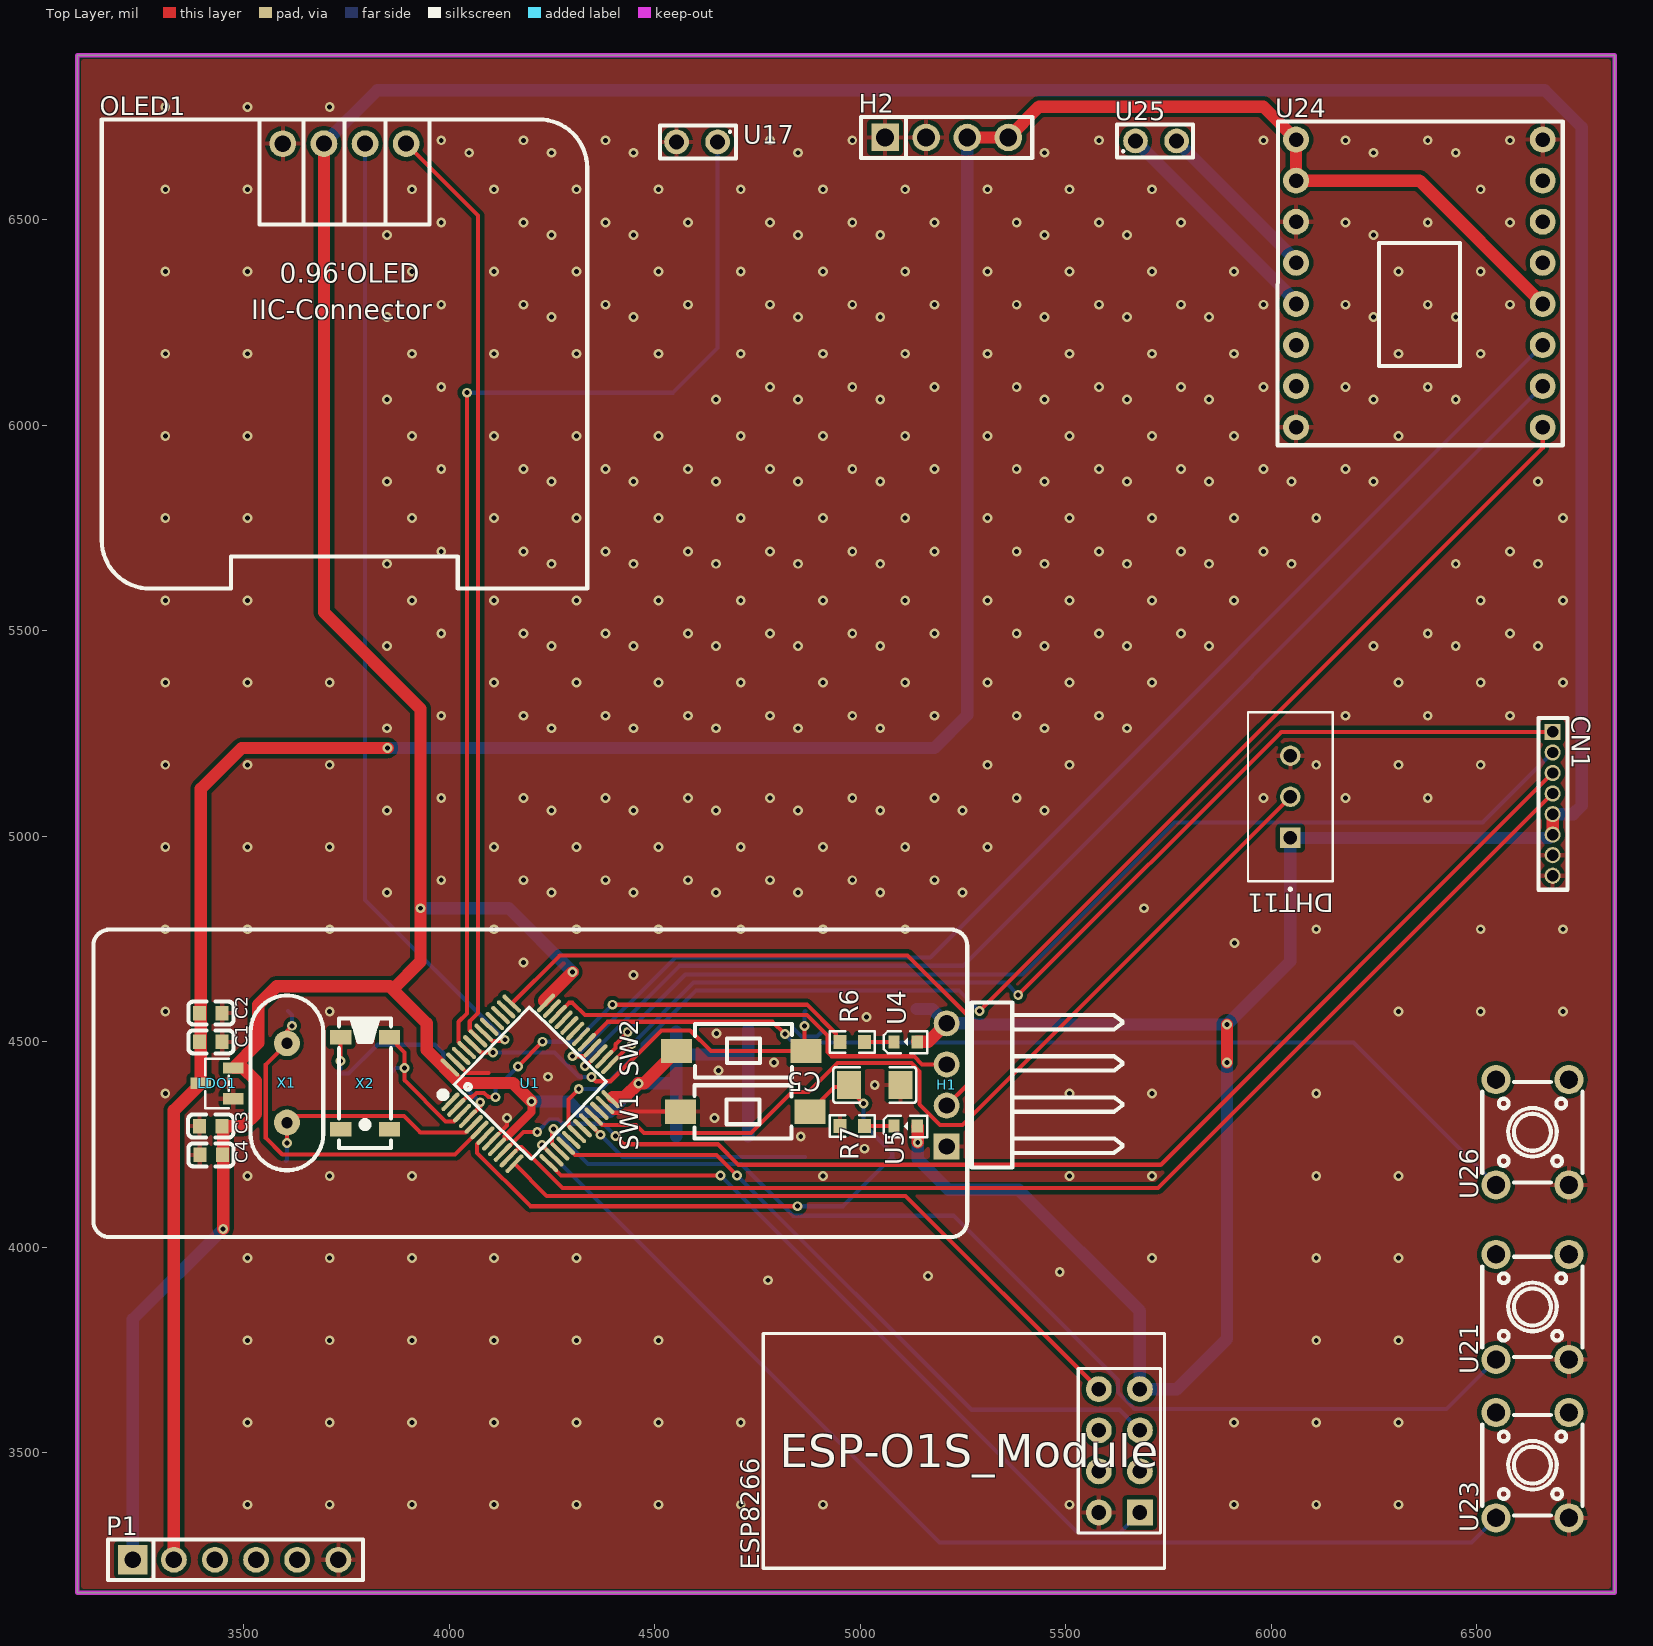
[diagram p0: Top Layer view]
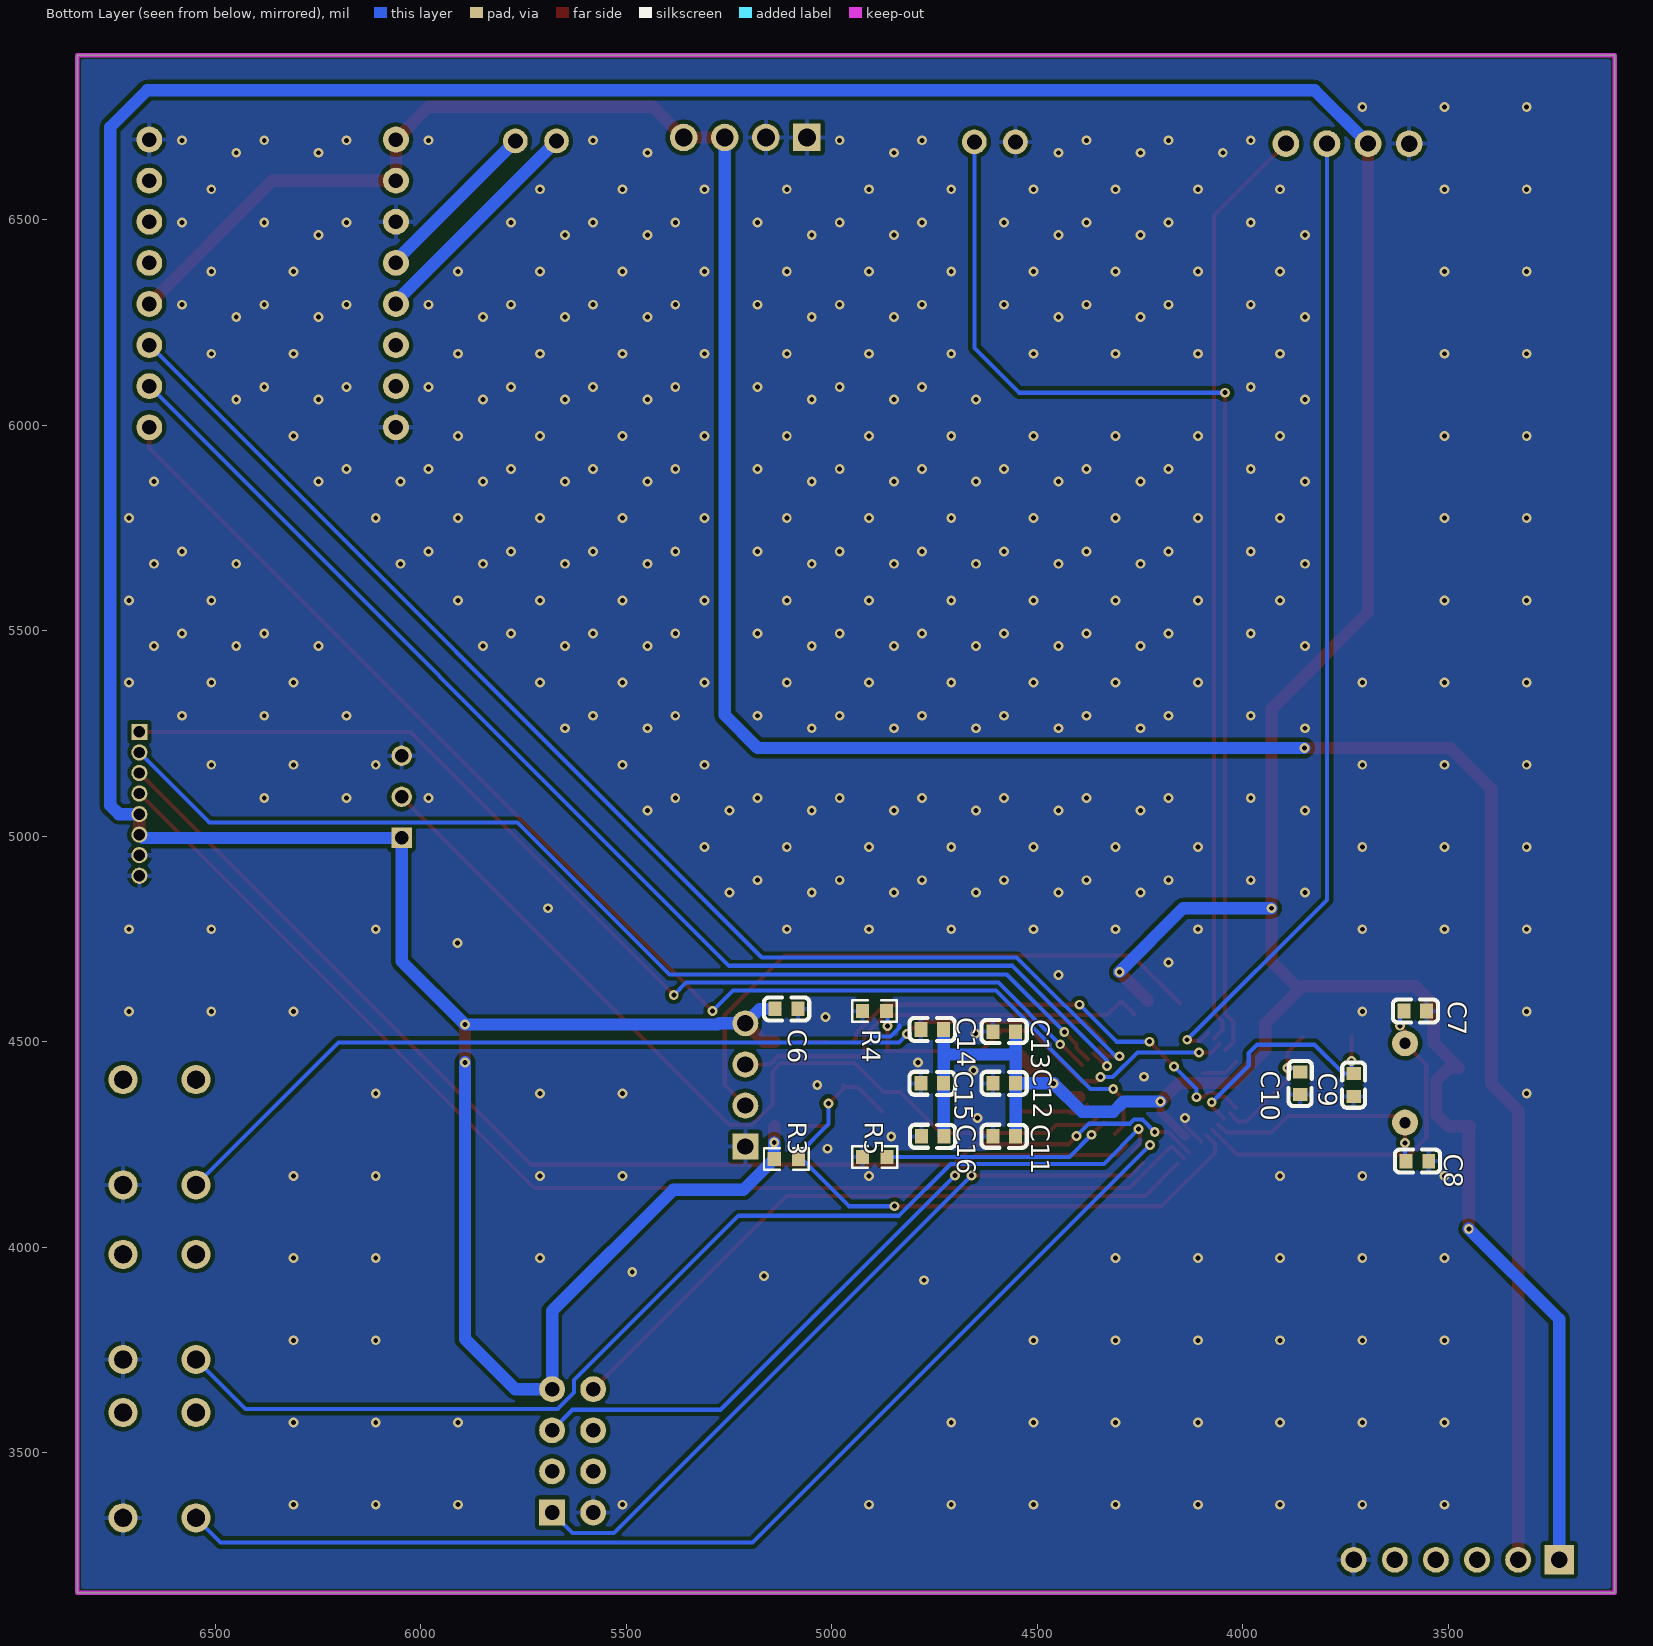
[diagram p1: Bottom Layer view, seen from below]
# Altium PCB MISC89131.pcbdoc
Units mil, origin at the board's own origin, x right, y up, seen from the top; angles counter-clockwise.
Board outline 3740.16 x 3740.16 mil, 2 copper layers (Top Layer, Bottom Layer), stack 62.206 mil thick; 42 components, 47 nets, 176 pads, 453 vias.

## Layer stack, top to bottom
Top Solder Mask Layer: solder mask 0.394, Dk 3.3
Top Layer: signal copper 1.379
Dielectric1: surface 59.449, FR4, Dk 4.5
Bottom Layer: signal copper 1.378
Bottom Solder Mask Layer: solder mask 0.394, Dk 3.3

## Board outline
3095,6900 3095,3159.84 6835.16,3159.84 6835.16,6900

## Design rules (kind name [scope] priority, off if disabled: settings)
BoardOutlineClearance copperThickness2oz_1 [All] p2: genericclearance=7.99 ignorepadtopadclearanceinfootprint=FALSE except(0: Arc-SplitContinuation Track-SplitContinuation SMDPad-SplitContinuation THPad-SplitContinuation Via-SplitContinuation Fill-SplitContinuation Region-SplitContinuation Poly-SplitContinuation Text-SplitContinuation Hole-SplitContinuation; 5.98: Arc-CutoutEdge Track-CutoutEdge SMDPad-CutoutEdge THPad-CutoutEdge Via-CutoutEdge Text-CutoutEdge; 6.89: Hole-OutlineEdge Hole-CutoutEdge; 10: Poly-OutlineEdge Poly-CutoutEdge; 11.81: Arc-OutlineEdge Track-OutlineEdge SMDPad-OutlineEdge THPad-OutlineEdge Via-OutlineEdge Fill-OutlineEdge Region-OutlineEdge Text-OutlineEdge Fill-CutoutEdge Region-CutoutEdge)
BoardOutlineClearance Plane_innerPlane_1 [All] p4 off: genericclearance=4.02 ignorepadtopadclearanceinfootprint=FALSE except(0: Arc-SplitContinuation Track-SplitContinuation SMDPad-SplitContinuation THPad-SplitContinuation Via-SplitContinuation Fill-SplitContinuation Region-SplitContinuation Poly-SplitContinuation Text-SplitContinuation Hole-SplitContinuation; 5.98: Arc-CutoutEdge Track-CutoutEdge SMDPad-CutoutEdge THPad-CutoutEdge Via-CutoutEdge Text-CutoutEdge; 6.89: Hole-OutlineEdge Hole-CutoutEdge; 10: Poly-OutlineEdge Poly-CutoutEdge; 11.81: Arc-OutlineEdge Track-OutlineEdge SMDPad-OutlineEdge THPad-OutlineEdge Via-OutlineEdge Fill-OutlineEdge Region-OutlineEdge Text-OutlineEdge Fill-CutoutEdge Region-CutoutEdge)
BoardOutlineClearance Copper_copperRegion_1 [All] p6 off: genericclearance=4.02 ignorepadtopadclearanceinfootprint=FALSE except(0: Arc-SplitContinuation Track-SplitContinuation SMDPad-SplitContinuation THPad-SplitContinuation Via-SplitContinuation Fill-SplitContinuation Region-SplitContinuation Poly-SplitContinuation Text-SplitContinuation Hole-SplitContinuation; 5.98: Arc-CutoutEdge Track-CutoutEdge SMDPad-CutoutEdge THPad-CutoutEdge Via-CutoutEdge Text-CutoutEdge; 6.89: Hole-OutlineEdge Hole-CutoutEdge; 10: Poly-OutlineEdge Poly-CutoutEdge; 11.81: Arc-OutlineEdge Track-OutlineEdge SMDPad-OutlineEdge THPad-OutlineEdge Via-OutlineEdge Fill-OutlineEdge Region-OutlineEdge Text-OutlineEdge Fill-CutoutEdge Region-CutoutEdge)
BoardOutlineClearance copperThickness1oz_1 [All] p8: genericclearance=4.02 ignorepadtopadclearanceinfootprint=FALSE except(0: Arc-SplitContinuation Track-SplitContinuation SMDPad-SplitContinuation THPad-SplitContinuation Via-SplitContinuation Fill-SplitContinuation Region-SplitContinuation Poly-SplitContinuation Text-SplitContinuation Hole-SplitContinuation; 5.98: Arc-CutoutEdge Track-CutoutEdge SMDPad-CutoutEdge THPad-CutoutEdge Via-CutoutEdge Text-CutoutEdge; 6.89: Hole-OutlineEdge Hole-CutoutEdge; 10: Poly-OutlineEdge Poly-CutoutEdge; 11.81: Arc-OutlineEdge Track-OutlineEdge SMDPad-OutlineEdge THPad-OutlineEdge Via-OutlineEdge Fill-OutlineEdge Region-OutlineEdge Text-OutlineEdge Fill-CutoutEdge Region-CutoutEdge)
Clearance copperThickness2oz [(InNet('+5V'))] p1: gap=7.99 ignorepadtopadclearanceinfootprint=FALSE except(5.98: SMDPad-Track SMDPad-SMDPad THPad-Track SMDPad-THPad THPad-THPad Track-Via SMDPad-Via THPad-Via Via-Via Fill-SMDPad Region-SMDPad Fill-THPad Region-THPad Fill-Via Region-Via Fill-Fill Fill-Region Region-Region Arc-Track Arc-SMDPad Arc-THPad Arc-Via Fill-Arc Region-Arc Arc-Arc Text-Track SMDPad-Text Text-THPad Text-Via Fill-Text Region-Text Arc-Text Text-Text; 6.89: Hole-Track Hole-SMDPad Hole-THPad Hole-Via Fill-Hole Region-Hole Hole-Arc Hole-Text; 10: Poly-Track Poly-SMDPad Poly-THPad Poly-Via Poly-Fill Poly-Region Poly-Poly Poly-Arc Poly-Text Poly-Hole; 11.81: Fill-Track Region-Track)
Clearance Plane_innerPlane [All] p3 off: gap=4.02 ignorepadtopadclearanceinfootprint=FALSE except(5.98: SMDPad-Track SMDPad-SMDPad THPad-Track SMDPad-THPad THPad-THPad Track-Via SMDPad-Via THPad-Via Via-Via Fill-SMDPad Region-SMDPad Fill-THPad Region-THPad Fill-Via Region-Via Fill-Fill Fill-Region Region-Region Arc-Track Arc-SMDPad Arc-THPad Arc-Via Fill-Arc Region-Arc Arc-Arc Text-Track SMDPad-Text Text-THPad Text-Via Fill-Text Region-Text Arc-Text Text-Text; 6.89: Hole-Track Hole-SMDPad Hole-THPad Hole-Via Fill-Hole Region-Hole Hole-Arc Hole-Text; 10: Poly-Track Poly-SMDPad Poly-THPad Poly-Via Poly-Fill Poly-Region Poly-Poly Poly-Arc Poly-Text Poly-Hole; 11.81: Fill-Track Region-Track)
Clearance Copper_copperRegion [All] p5 off: gap=4.02 ignorepadtopadclearanceinfootprint=FALSE except(5.98: SMDPad-Track SMDPad-SMDPad THPad-Track SMDPad-THPad THPad-THPad Track-Via SMDPad-Via THPad-Via Via-Via Fill-SMDPad Region-SMDPad Fill-THPad Region-THPad Fill-Via Region-Via Fill-Fill Fill-Region Region-Region Arc-Track Arc-SMDPad Arc-THPad Arc-Via Fill-Arc Region-Arc Arc-Arc Text-Track SMDPad-Text Text-THPad Text-Via Fill-Text Region-Text Arc-Text Text-Text; 6.89: Hole-Track Hole-SMDPad Hole-THPad Hole-Via Fill-Hole Region-Hole Hole-Arc Hole-Text; 10: Poly-Track Poly-SMDPad Poly-THPad Poly-Via Poly-Fill Poly-Region Poly-Poly Poly-Arc Poly-Text Poly-Hole; 11.81: Fill-Track Region-Track)
Clearance copperThickness1oz [All] p7: gap=4.02 ignorepadtopadclearanceinfootprint=FALSE except(5.98: SMDPad-Track SMDPad-SMDPad THPad-Track SMDPad-THPad THPad-THPad Track-Via SMDPad-Via THPad-Via Via-Via Fill-SMDPad Region-SMDPad Fill-THPad Region-THPad Fill-Via Region-Via Fill-Fill Fill-Region Region-Region Arc-Track Arc-SMDPad Arc-THPad Arc-Via Fill-Arc Region-Arc Arc-Arc Text-Track SMDPad-Text Text-THPad Text-Via Fill-Text Region-Text Arc-Text Text-Text; 6.89: Hole-Track Hole-SMDPad Hole-THPad Hole-Via Fill-Hole Region-Hole Hole-Arc Hole-Text; 10: Poly-Track Poly-SMDPad Poly-THPad Poly-Via Poly-Fill Poly-Region Poly-Poly Poly-Arc Poly-Text Poly-Hole; 11.81: Fill-Track Region-Track)
DiffPairsRouting differentialPair [All] p1: maxlimit=6 minlimit=6 mostfreqgap=6 toplayer_minwidth=5 toplayer_prefwidth=10 toplayer_maxwidth=100 toplayer_mingap=6 toplayer_prefgap=6 toplayer_maxgap=6 bottomlayer_minwidth=5 bottomlayer_prefwidth=10 bottomlayer_maxwidth=100 bottomlayer_mingap=6 bottomlayer_prefgap=6 bottomlayer_maxgap=6 maxuncoupledlength=10
HoleToHoleClearance otherClearance [All] p1: gap=11.81 allowstackedmicrovias=TRUE
Length netLength [All] p1: minlimit=0 maxlimit=0
PasteMaskExpansion pasteMaskExpansion [All] p1: expansion=0
PlaneConnect innerPlane [All] p1: planeconnectstyle=Relief reliefexpansion=20 reliefentries=4 reliefconductorwidth=10 reliefairgap=10
PolygonConnect copperRegion [All] p1: connectstyle=Relief reliefconductorwidth=10 reliefentries=4 polygonreliefangle="90 Angle" airgapwidth=10 via.connectstyle=Relief via.reliefconductorwidth=10 via.reliefentries=4 via.polygonreliefangle="90 Angle" via.airgapwidth=10
RoutingVias viaSize [All] p1: holewidth=12.01 width=24.02 viastyle="Through Hole" minholewidth=11.81 minwidth=19.68 maxholewidth=248.03 maxwidth=393.7
SolderMaskExpansion solderMaskExpansion [IsVia] p1: expansion=-1000 istentingtop=TRUE
SolderMaskExpansion solderMaskExpansion [All] p2: expansion=2.01 istentingtop=FALSE
Width copperThickness2oz_2 [(InNet('+5V'))] p1: maxlimit=100 minlimit=15 preferedwidth=15
Width copperThickness1oz_2 [All] p2: maxlimit=100 minlimit=5 preferedwidth=10

## Components (designator, comment, footprint, x,y, rotation, side; value= is the part's Value field where it differs from the comment)
C1 "10uF" C0603 3420,4500 r180 top
C2 "100nF" C0603 3420,4570 r180 top
C3 "100nF" C0603 3420,4295 r0 top
C4 "10uF" C0603 3420.61,4224.79 r0 top
C5 "100uF" C1206 5035,4395 r180 top
C6 "100nF" C0603 5109.76,4580 r0 bottom
C7 "20pF" C0603 3580,4575 r0 bottom
C8 "20pF" C0603 3575,4210 r0 bottom
C9 "20pF" C0603 3730,4395 r90 bottom
C10 "20pF" C0603 3860,4399.02 r90 bottom
C11 "100nF" C0603 4580,4270 r180 bottom
C12 "100nF" C0603 4580,4399.02 r180 bottom
C13 "100nF" C0603 4580,4525 r180 bottom
C14 "100nF" C0603 4755,4530 r180 bottom
C15 "100nF" C0603 4755,4399.02 r180 bottom
C16 "4.7nF" C0603 4754.05,4270 r180 bottom
CN1 "2.0mm*8P female header" HDR-TH_8P-P1.27_2.0MM-8P 6684.01,5079.02 r270 top
DHT11 "" PIN3直插DHT11 6135,5085 r180 top
ESP8266 "" ESP8266-01S_Module 5630,3505 r90 top
H1 "A254AD-WD04P" HDR-TH_4P-P2.54-H-M-W10.2 5210,4395 r90 top
H2 "4P" HDR-TH_4P-P2.54-V-M-3 5210,6700 r0 top
LDO1 "SC662K-3.3V" SOT-23-3_L2.9-W1.3-P1.90-LS2.4-BR 3435,4399.02 r0 top
OLED1 "" 0.96OLED_4P 3745,6685 r0 top
P1 "MINI USB power input module" HDR-TH_6P-P2.54-V-F 3480,3240 r0 top
R3 "1kΩ" R0603 5110,4215 r0 bottom
R4 "10kΩ" R0603 4895.68,4575 r180 bottom
R5 "10kΩ" R0603 4895,4220 r180 bottom
R6 "510Ω" R0603 4980,4500 r180 top
R7 "510Ω" R0603 4980,4295 r180 top
SW1 "TS-1101-C-W" SW-SMD_L6.0-W3.3-LS8.0 4720,4330.12 r0 top
SW2 "TS-1101-C-W" SW-SMD_L6.0-W3.3-LS8.0 4710,4477.76 r180 top
U1 "STM32F103C8T6" LQFP-48_L7.0-W7.0-P0.50-LS9.0-BL 4197.01,4399.02 r316 top
U4 "42-51/GHC-YW2X2K/3T" LED-SMD_L1.6-W0.8-FD_GREEN-1 5110,4500 r180 top
U5 "42-51/GHC-YW2X2K/3T" LED-SMD_L1.6-W0.8-FD_GREEN-1 5110,4295 r180 top
U17 "" 2p排针 4652.81,6689.16 r180 top
U21 "UP" KEY-TH_4P复位按键 6635,3855 r90 top
U23 "DOWN" KEY-TH_4P复位按键 6635,3470 r90 top
U24 "" TB6612电机驱动 6360,6345 r0 top
U25 "" 2p排针 5669.39,6691.55 r0 top
U26 "UP" KEY-TH_4P复位按键 6635,4280 r90 top
X1 "8MHz" OSC-TH_L10.0-W4.5-P5.00 3605,4400 r180 top
X2 "32.768kHz" MC-306_4P-L8.0-W3.2-P5.5-BL 3795,4399.02 r270 top

## Footprints (in the part's own frame and the unit in brackets; to place one, negate y for a bottom-side part, rotate by r counter-clockwise, add the part's x,y. Pads: shape width x height; smd on the part's side, far side on the other; paste and mask are expansions set on the pad)
0.96OLED_4P [mm]
  round 1.65 hole 1 copper offset 0,0: 1(-3.81,-0.001) 2(-1.27,0.002) 3(1.27,0.002) 4(3.81,0.002)
  silkscreen extent -15,-27.5 15,1.5
2p排针 [mil]
  round 60 hole 36: 1(0,0) 2(100,0)
  silkscreen extent -45,-40 140,40
C0603 [mm]
  rect 0.8x0.9 smd: 1(-0.7,0) 2(0.7,0)
  silkscreen extent -1.41,-0.71 1.39,0.72
C1206 [mm]
  rect 1.485x1.728 smd paste-100 mask+0.051: 1(-1.593,0) 2(1.593,0)
  silkscreen extent -2.56,-1.09 2.56,1.09
ESP8266-01S_Module [mm]
  rect 1.6x1.6 hole 0.9: 1(-3.81,-1.27)
  round 1.6 hole 0.9: 2(-3.81,1.27) 3(-1.27,-1.27) 4(-1.27,1.27) 5(1.27,-1.27) 6(1.27,1.27) 7(3.81,-1.27) 8(3.81,1.27)
  silkscreen extent -7.25,-2.79 7.25,22.01
HDR-TH_4P-P2.54-H-M-W10.2 [mm]
  rect 1.6x1.6 hole 1: 1(-3.81,0)
  round 1.6 hole 1: 2(-1.27,0) 3(1.27,0) 4(3.81,0)
  silkscreen extent -5.1,-10.85 5.1,-1.55
HDR-TH_4P-P2.54-V-M-3 [mil]
  rect 66.9x66.9 hole 43.3 paste+0 mask+2: 1(-150,0)
  round 66.9 hole 43.3 paste+0 mask+2: 2(-50,0) 3(50,0) 4(150,0)
  silkscreen extent -208,-50 208,50
HDR-TH_6P-P2.54-V-F [mm]
  rect 1.8x1.8 hole 1.02: 1(-6.35,0)
  round 1.6 hole 1.02: 2(-3.81,0) 3(-1.27,0) 4(1.27,0) 5(3.81,0) 6(6.35,0)
  silkscreen extent -7.87,-1.25 7.87,1.25
HDR-TH_8P-P1.27_2.0MM-8P [mm]
  rect 1x1 hole 0.7: 1(-4.445,0)
  round 1 hole 0.7: 2(-3.175,0) 3(-1.905,0) 4(-0.635,0) 5(0.635,0) 6(1.905,0) 7(3.175,0) 8(4.445,0)
  silkscreen extent -5.31,-0.87 5.31,0.92
KEY-TH_4P复位按键 [mm]
  round 1.8 hole 1.1 slot 1.105 at 0 deg: 1(-3.251,2.25) 2(3.251,2.25) 3(-3.251,-2.25) 4(3.251,-2.25)
  silkscreen extent -3.1,-3.1 3.1,3.1
LED-SMD_L1.6-W0.8-FD_GREEN-1 [mm]
  rect 0.7x0.8 smd: 1(-0.715,0) 2(0.715,0)
  silkscreen extent -1.35,-0.65 1.35,0.7
LQFP-48_L7.0-W7.0-P0.50-LS9.0-BL [mm]
  oval 0.27x1.5 smd rot 179.96 paste+0 mask+0.05: 1(-2.753,-4.248) 2(-2.253,-4.248) 3(-1.753,-4.249) 4(-1.253,-4.249) 5(-0.753,-4.249) 6(-0.253,-4.25) 7(0.247,-4.25) 8(0.747,-4.25) 9(1.247,-4.251) 10(1.747,-4.251) 11(2.247,-4.251) 12(2.747,-4.252) 25(2.753,4.248) 26(2.253,4.248) 27(1.753,4.249) 28(1.253,4.249) 29(0.753,4.249) 30(0.253,4.25) 31(-0.247,4.25) 32(-0.747,4.25) 33(-1.247,4.251) 34(-1.747,4.251) 35(-2.247,4.251) 36(-2.747,4.252)
  oval 1.5x0.27 smd rot 179.96 paste+0 mask+0.05: 13(4.248,-2.753) 14(4.248,-2.253) 15(4.249,-1.753) 16(4.249,-1.253) 17(4.249,-0.753) 18(4.25,-0.253) 19(4.25,0.247) 20(4.25,0.747) 21(4.251,1.247) 22(4.251,1.747) 23(4.251,2.247) 24(4.252,2.747) 37(-4.248,2.753) 38(-4.248,2.253) 39(-4.249,1.753) 40(-4.249,1.253) 41(-4.249,0.753) 42(-4.25,0.253) 43(-4.25,-0.247) 44(-4.25,-0.747) 45(-4.251,-1.247) 46(-4.251,-1.747) 47(-4.251,-2.247) 48(-4.252,-2.747)
  silkscreen extent -3.59,-4.46 3.3,3.34
MC-306_4P-L8.0-W3.2-P5.5-BL [mm]
  rect 0.9x1.3 smd: 1(-2.85,-1.5) 2(2.85,-1.5) 3(2.85,1.5) 4(-2.85,1.5)
  silkscreen extent -4,-1.6 4,1.6
OSC-TH_L10.0-W4.5-P5.00 [mm]
  round 1.6 hole 0.7: 1(0,2.45) 2(0,-2.45)
  silkscreen extent -2.25,-5.39 2.25,5.39
PIN3直插DHT11 [mm]
  rect 1.26x1.26 hole 0.84: 1(2.26,2.26)
  round 1.26 hole 0.84: 2(2.26,-0.28) 3(2.26,-2.82)
  silkscreen extent -0.36,-5.51 4.88,5.51
R0603 [mil]
  rect 31.75x34.02 smd paste-3937.01 mask+2: 1(-29.66,0) 2(29.66,0)
  silkscreen extent -55,-26 55,26
SOT-23-3_L2.9-W1.3-P1.90-LS2.4-BR [mm]
  rect 1.25x0.7 smd: 1(1,-0.95) 2(1,0.95) 3(-1,0)
  silkscreen extent -0.73,-1.53 0.73,1.53
SW-SMD_L6.0-W3.3-LS8.0 [mm]
  rect 1.9x1.5 smd: 1(-4,0) 2(4,0)
  silkscreen extent -3.14,-1.67 2.86,1.63
TB6612电机驱动 [mm]
  round 1.6 hole 0.9 paste+0 mask+0.051: 1(-7.62,8.89) 2(-7.62,6.35) 3(-7.62,3.81) 4(-7.62,1.27) 5(-7.62,-1.27) 6(-7.62,-3.81) 7(-7.62,-6.35) 8(-7.62,-8.89) 9(7.62,8.89) 10(7.62,6.35) 11(7.62,3.81) 12(7.62,1.27) 13(7.62,-1.27) 14(7.62,-3.81) 15(7.62,-6.35) 16(7.62,-8.89)
  silkscreen extent -8.77,-10 8.86,10

## Via types
v1: diameter 24.02, hole 12, Top Layer to Bottom Layer, 453 vias

## Nets (pads, with @x,y where several pads share a name; then routed paths per layer and width w, separated by ;. In a path a pad name is that pad's centre, name@x,y a point inside that pad or via, vN(x,y) a via of type N, cw(c..) or ccw(c..) an arc to the next point about the centre after c; other vN are vias at no path point)
3V3: C3.2 C4.2 C6.2 C11.2 C12.2 C13.2 C14.2 C15.2 C16.2 CN1.5 CN1.6 DHT11.1 ESP8266.7 H1.4 LDO1.2 OLED1.2 P1.1 R3.2 SW2.2 U1.9 U1.24 U1.36 U1.48 U4.1 U5.1 | length 15462.2
  Top Layer w20: 4139.99,4269.54 4200,4329.55 v1(4200,4355)
  Top Layer w30: v1(3450,4045) 3450,4292.56 C3.2 3500,4295 3529.6,4324.6 3529.6,4405.4 3498.58,4436.42 LDO1.2 3535,4497.05 3535,4590 3580,4635 3855,4635 3862.5,4627.5 ; OLED1.2@3695,6685.05 3695,5545 3930,5310 v1(3930,4825) 3930,4695 3862.5,4627.5 ; v1(4200,4355) 4155.05,4399.95 4025.05,4399.95 3945,4480 3945,4545 3862.5,4627.5 ; 4230.53,4599.52 4230.53,4600.53 v1(4300,4670) ; 4397.51,4365.49 4426.48,4365.49 v1(4460,4399.02) 4473.78,4399.02 SW2.2 ; U5.1 5139.66,4293.49 v1(5139.66,4255) ; U4.1 5165,4500 H1.4 ; v1(5892.01,4450) v1(5892.01,4542.01) ; CN1.6 CN1.5
  Bottom Layer w30: P1.1 3230,3825 v1(3450,4045) ; OLED1.2@3695,6685.05 3824.95,6815 6665,6815 6755,6725 6755,5075 6734.02,5054.02 CN1.5 ; v1(3930,4825) 4145,4825 v1(4300,4670) ; v1(4200,4355) 4290,4355 4315,4330 4390.98,4330 v1(4460,4399.02) C12.2 ; C11.2 C12.2 ; C13.2 4552.44,4469.33 ; C16.2 4727.44,4270.95 C15.2 4727.44,4462.17 ; C14.2 4727.44,4462.17 ; C6.2 5175,4580 H1.4 5273.34,4545 5276.33,4542.01 v1(5892.01,4542.01) 6046.02,4696.02 DHT11.1 6676.01,4996.02 CN1.6 ; v1(5139.66,4255) R3.2 5214.66,4140 5385,4140 5680,3845 ESP8266.7 5770,3655 5892.01,3777.01 v1(5892.01,4450) ; C12.2 4552.44,4469.33 ; 4552.44,4469.33 4720.27,4469.33 4727.44,4462.17
$1N3910: R6.1 U4.2 | length 72.2
  Top Layer w10: R6.1 U4.2
$1N3911: R7.1 U5.2 | length 72.2
  Top Layer w10: R7.1 U5.2
+5V: C1.2 C2.2 H2.3 H2.4 LDO1.3 P1.2 U24.1 U24.2 U24.13 | length 6934.9
  Top Layer w30: P1.2 3330,4333.39 LDO1.3 3395.63,5115.63 3495,5215 v1(3850,5215) ; H2.3 H2.4 5435,6775 5980,6775 U24.1 U24.2 6360,6595 U24.13
  Bottom Layer w30: v1(3850,5215) 5180,5215 5260,5295 H2.3
AO1: U24.4 U25.2 | length 416.9
  Bottom Layer w30: U25.2 6060,6400.94 U24.4
AO2: U24.5 U25.1 | length 558.3
  Bottom Layer w30: U25.1 6060,6300.94 U24.5
BOOT0: R4.2 SW2.1 U1.44 | length 1020
  Top Layer w10: U1.44 4076.2,4474.1 v1(4106.2,4474.1) ; v1(4346.2,4414.1) 4356.2,4404.1 4392.54,4404.1 4516.2,4527.76 4586.2,4527.76 4636.2,4477.76 SW2.1 4863.98,4481.26 v1(4863.98,4538.51)
  Bottom Layer w10: v1(4106.2,4474.1) 4256.2,4474.1 4316.2,4414.1 v1(4346.2,4414.1) ; v1(4863.98,4538.51) 4863.98,4572.96 R4.2
BOOT1: R5.2 U1.20 | length 562.3
  Top Layer w10: U1.20 v1(4367.81,4273.93)
  Bottom Layer w10: v1(4367.81,4273.93) 4421.74,4220 R5.2
CLK: H1.2 U1.37 | length 1457.2
  Top Layer w10: U1.37 4268.83,4710 5115,4710 5260,4565 5260,4395 H1.2
DIO: H1.3 U1.34 | length 1043.3
  Top Layer w10: U1.34 4291.6,4595 4300,4595 4330,4565 4870,4565 4920,4515 4920,4475 4930,4465 5130,4465 5150,4445 H1.3
GND: C1.1 C2.1 C3.1 C4.1 C5.1 C6.1 C7.1 C8.1 C9.1 C10.1 C11.1 C12.1 C13.1 C14.1 C15.1 C16.1 CN1.7 CN1.8 DHT11.3 ESP8266.2 H1.1 H2.1 H2.2 LDO1.1 OLED1.1 P1.6 R4.1 R5.1 R7.2 SW1.1 U1.8 U1.23 U1.35 U1.47 U17.2 U21.3 U23.3 U24.3 U24.8 U24.9 U26.3 | length 446.5
  Top Layer w10: U1.47 4042.83,4423.97 4095,4423.97 ; U1.8 4120.98,4277.26 4120.98,4277.42 4140,4296.45 v1(4140,4315) ; U1.23 4397.84,4327.4 4416.71,4327.4 4419.42,4330.12 SW1.1
  Bottom Layer w10: 4835,4540 4835,4534.97 4857.19,4512.78 4895,4512.78 4906.11,4523.89
  other v1: 3509.1,3373.94 3709.1,3373.94 3909.1,3373.94 4109.1,3373.94 4309.1,3373.94 4509.1,3373.94 4709.1,3373.94 4909.1,3373.94 5509.1,3373.94 5909.1,3373.94 6109.1,3373.94 6309.1,3373.94 3509.1,3573.94 3709.1,3573.94 3909.1,3573.94 4109.1,3573.94 4309.1,3573.94 4509.1,3573.94 4709.1,3573.94 5909.1,3573.94 6109.1,3573.94 6309.1,3573.94 3509.1,3773.94 3709.1,3773.94 3909.1,3773.94 4109.1,3773.94 4309.1,3773.94 4509.1,3773.94 6109.1,3773.94 6309.1,3773.94 4775,3920 5165,3930 5485,3940 3509.1,3973.94 3709.1,3973.94 3909.1,3973.94 4109.1,3973.94 4309.1,3973.94 5709.1,3973.94 6109.1,3973.94 6309.1,3973.94 3509.1,4173.94 3709.1,4173.94 3909.1,4173.94 4909.1,4173.94 5509.1,4173.94 5709.1,4173.94 6109.1,4173.94 6309.1,4173.94 5010,4240 4855,4270 4645,4315 3309.1,4373.94 5509.1,4373.94 5709.1,4373.94 6109.1,4373.94 5035,4395 4240,4415 4655,4430 4790,4450 4650,4520 5015,4560 3309.1,4573.94 3709.1,4573.94 6309.1,4573.94 6509.1,4573.94 6709.1,4573.94 4448.42,4662.9 4180.38,4693.2 5910,4740 3309.1,4773.94 3509.1,4773.94 3709.1,4773.94 4109.1,4773.94 4309.1,4773.94 4509.1,4773.94 4709.1,4773.94 4909.1,4773.94 5109.1,4773.94 6109.1,4773.94 6509.1,4773.94 6709.1,4773.94 5690,4825 3848.42,4862.9 4248.42,4862.9 4448.42,4862.9 4648.42,4862.9 4848.42,4862.9 5048.42,4862.9 5248.42,4862.9 3980.38,4893.2 4180.38,4893.2 4380.38,4893.2 4580.38,4893.2 4780.38,4893.2 4980.38,4893.2 5180.38,4893.2 3309.1,4973.94 3509.1,4973.94 3709.1,4973.94 4109.1,4973.94 4309.1,4973.94 4509.1,4973.94 4709.1,4973.94 4909.1,4973.94 5109.1,4973.94 5309.1,4973.94 3848.42,5062.9 4248.42,5062.9 4448.42,5062.9 4648.42,5062.9 4848.42,5062.9 5048.42,5062.9 5248.42,5062.9 5448.42,5062.9 3980.38,5093.2 4180.38,5093.2 4380.38,5093.2 4580.38,5093.2 4780.38,5093.2 4980.38,5093.2 5180.38,5093.2 5380.38,5093.2 5980.38,5093.2 6180.38,5093.2 6380.38,5093.2 3309.1,5173.94 3509.1,5173.94 3709.1,5173.94 5309.1,5173.94 5509.1,5173.94 6109.1,5173.94 6309.1,5173.94 6509.1,5173.94 3848.42,5262.9 4248.42,5262.9 4448.42,5262.9 4648.42,5262.9 4848.42,5262.9 5048.42,5262.9 5448.42,5262.9 5648.42,5262.9 3980.38,5293.2 4180.38,5293.2 4380.38,5293.2 4580.38,5293.2 4780.38,5293.2 4980.38,5293.2 5180.38,5293.2 5380.38,5293.2 5580.38,5293.2 6180.38,5293.2 6380.38,5293.2 6580.38,5293.2 3309.1,5373.94 3509.1,5373.94 3709.1,5373.94 4109.1,5373.94 4309.1,5373.94 4509.1,5373.94 4709.1,5373.94 4909.1,5373.94 5109.1,5373.94 5309.1,5373.94 5509.1,5373.94 5709.1,5373.94 6309.1,5373.94 6509.1,5373.94 6709.1,5373.94 3848.42,5462.9 4248.42,5462.9 4448.42,5462.9 4648.42,5462.9 4848.42,5462.9 5048.42,5462.9 5448.42,5462.9 5648.42,5462.9 5848.42,5462.9 6248.42,5462.9 6448.42,5462.9 6648.42,5462.9 3980.38,5493.2 4180.38,5493.2 4380.38,5493.2 4580.38,5493.2 4780.38,5493.2 4980.38,5493.2 5180.38,5493.2 5380.38,5493.2 5580.38,5493.2 5780.38,5493.2 6380.38,5493.2 6580.38,5493.2 3309.1,5573.94 3509.1,5573.94 3909.1,5573.94 4109.1,5573.94 4309.1,5573.94 4509.1,5573.94 4709.1,5573.94 4909.1,5573.94 5109.1,5573.94 5309.1,5573.94 5509.1,5573.94 5709.1,5573.94 5909.1,5573.94 6509.1,5573.94 6709.1,5573.94 3848.42,5662.9 4248.42,5662.9 4448.42,5662.9 4648.42,5662.9 4848.42,5662.9 5048.42,5662.9 5448.42,5662.9 5648.42,5662.9 5848.42,5662.9 6048.42,5662.9 6448.42,5662.9 6648.42,5662.9 3980.38,5693.2 4180.38,5693.2 4380.38,5693.2 4580.38,5693.2 4780.38,5693.2 4980.38,5693.2 5180.38,5693.2 5380.38,5693.2 5580.38,5693.2 5780.38,5693.2 5980.38,5693.2 6580.38,5693.2 3309.1,5773.94 3509.1,5773.94 3909.1,5773.94 4109.1,5773.94 4309.1,5773.94 4509.1,5773.94 4709.1,5773.94 4909.1,5773.94 5109.1,5773.94 5309.1,5773.94 5509.1,5773.94 5709.1,5773.94 5909.1,5773.94 6109.1,5773.94 6709.1,5773.94 3848.42,5862.9 4248.42,5862.9 4448.42,5862.9 4648.42,5862.9 4848.42,5862.9 5048.42,5862.9 5448.42,5862.9 5648.42,5862.9 5848.42,5862.9 6048.42,5862.9 6248.42,5862.9 6648.42,5862.9 3980.38,5893.2 4180.38,5893.2 4380.38,5893.2 4580.38,5893.2 4780.38,5893.2 4980.38,5893.2 5180.38,5893.2 5380.38,5893.2 5580.38,5893.2 5780.38,5893.2 5980.38,5893.2 6180.38,5893.2 3309.1,5973.94 3509.1,5973.94 3909.1,5973.94 4109.1,5973.94 4309.1,5973.94 4509.1,5973.94 4709.1,5973.94 4909.1,5973.94 5109.1,5973.94 5309.1,5973.94 5509.1,5973.94 5709.1,5973.94 5909.1,5973.94 6309.1,5973.94 3848.42,6062.9 4648.42,6062.9 4848.42,6062.9 5048.42,6062.9 5448.42,6062.9 5648.42,6062.9 5848.42,6062.9 6248.42,6062.9 6448.42,6062.9 3980.38,6093.2 4780.38,6093.2 4980.38,6093.2 5180.38,6093.2 5380.38,6093.2 5580.38,6093.2 5780.38,6093.2 5980.38,6093.2 6180.38,6093.2 6380.38,6093.2 3309.1,6173.94 3509.1,6173.94 3909.1,6173.94 4109.1,6173.94 4309.1,6173.94 4509.1,6173.94 4709.1,6173.94 4909.1,6173.94 5109.1,6173.94 5309.1,6173.94 5509.1,6173.94 5709.1,6173.94 5909.1,6173.94 6309.1,6173.94 6509.1,6173.94 3848.42,6262.9 4248.42,6262.9 4448.42,6262.9 4848.42,6262.9 5048.42,6262.9 5448.42,6262.9 5648.42,6262.9 5848.42,6262.9 6248.42,6262.9 6448.42,6262.9 3980.38,6293.2 4180.38,6293.2 4380.38,6293.2 4580.38,6293.2 4780.38,6293.2 4980.38,6293.2 5180.38,6293.2 5380.38,6293.2 5580.38,6293.2 5780.38,6293.2 5980.38,6293.2 6180.38,6293.2 6380.38,6293.2 6580.38,6293.2 3309.1,6373.94 3509.1,6373.94 3909.1,6373.94 4109.1,6373.94 4309.1,6373.94 4509.1,6373.94 4709.1,6373.94 4909.1,6373.94 5109.1,6373.94 5309.1,6373.94 5509.1,6373.94 5709.1,6373.94 5909.1,6373.94 6309.1,6373.94 6509.1,6373.94 3848.42,6462.9 4248.42,6462.9 4448.42,6462.9 4848.42,6462.9 5048.42,6462.9 5448.42,6462.9 5648.42,6462.9 6248.42,6462.9 3980.38,6493.2 4180.38,6493.2 4380.38,6493.2 4580.38,6493.2 4780.38,6493.2 4980.38,6493.2 5180.38,6493.2 5380.38,6493.2 5580.38,6493.2 5780.38,6493.2 6180.38,6493.2 6380.38,6493.2 6580.38,6493.2 3309.1,6573.94 3509.1,6573.94 3909.1,6573.94 4109.1,6573.94 4309.1,6573.94 4509.1,6573.94 4709.1,6573.94 4909.1,6573.94 5109.1,6573.94 5309.1,6573.94 5509.1,6573.94 5709.1,6573.94 6509.1,6573.94 4048.42,6662.9 4248.42,6662.9 4448.42,6662.9 4848.42,6662.9 5448.42,6662.9 6248.42,6662.9 6448.42,6662.9 3980.38,6693.2 4180.38,6693.2 4380.38,6693.2 4780.38,6693.2 4980.38,6693.2 5580.38,6693.2 5980.38,6693.2 6180.38,6693.2 6380.38,6693.2 6580.38,6693.2 3309.1,6773.94 3509.1,6773.94 3709.1,6773.94
OSC32-IN: C10.2 U1.3 X2.4 | length 345
  Top Layer w10: X2.4 3891.16,4474.11 v1(3891.16,4436.63) 3891.16,4406.63 3991.16,4306.63 4011.16,4306.63 U1.3
  Bottom Layer w10: C10.2 3870.06,4436.63 v1(3891.16,4436.63)
OSC32-OUT: C9.2 U1.4 X2.1 | length 590.8
  Top Layer w10: v1(3735.32,4452.95) 3735.32,4510.59 X2.1 ; U1.4 4075.32,4342.95 v1(4075.32,4352.95)
  Bottom Layer w10: C9.2 C9.2@3735.32,4422.95 ; v1(3735.32,4452.95) C9.2@3735.32,4422.95 ; v1(4075.32,4352.95) 3985.32,4442.95 3985.32,4472.95 3965.32,4492.95 3825.32,4492.95 3755.32,4422.95 C9.2@3735.32,4422.95
OSC-IN: C8.2 U1.5 X1.1 | length 580.4
  Top Layer w10: v1(3605,4253.54) X1.1 3620.72,4319.26 3889.46,4319.26 3929.46,4279.26 4039.46,4279.26 U1.5
  Bottom Layer w10: C8.2 3605,4212.44 v1(3605,4253.54)
OSC-OUT: C7.2 U1.6 X1.2 | length 901.5
  Top Layer w10: v1(3617.56,4539.02) 3605,4526.46 X1.2 3553.62,4445.08 3553.62,4265.58 3593.62,4225.58 4013.62,4225.58 U1.6
  Bottom Layer w10: C7.2 3617.56,4565 v1(3617.56,4539.02)
PA0: CN1.3 U1.10 | length 3027.3
  Top Layer w10: U1.10 4180.22,4280.84 v1(4214.01,4280.84) ; v1(4404.01,4270.84) 4424.01,4250.84 4654.01,4250.84 4704.01,4200.84 5730.83,4200.84 CN1.3
  Bottom Layer w10: v1(4214.01,4280.84) 4244.01,4310.84 4264.01,4310.84 4274.01,4300.84 4374.01,4300.84 v1(4404.01,4270.84)
PA1: CN1.4 U1.11 | length 2989.8
  Top Layer w10: U1.11 4171.23,4244.02 4175.55,4244.02 4275.55,4144.02 5724.01,4144.02 CN1.4
PA2: ESP8266.8 U1.12 | length 1648.7
  Top Layer w10: U1.12 4236.99,4125 5110,4125 ESP8266.8
PA3: ESP8266.1 U1.13 | length 1831.4
  Top Layer w10: U1.13 4271.89,4175 v1(4660,4175)
  Bottom Layer w10: v1(4660,4175) 5530,3305 5630,3305 ESP8266.1
PA4: U1.14 U23.1 | length 2788.5
  Top Layer w10: v1(4225.71,4249.03) U1.14
  Bottom Layer w10: v1(4225.71,4249.03) 5192.73,3282 6486.4,3282 U23.1
PA5: U1.15 U21.1 | length 2706.6
  Top Layer w10: v1(4253.22,4287.53) 4249.39,4283.7 4249.39,4253.17 U1.15
  Bottom Layer w10: v1(4253.22,4287.53) 4337.57,4203.17 4710.23,4203.17 4836.4,4077 5226.4,4077 5626.4,3677 5626.4,3647 5666.4,3607 6426.4,3607 U21.1
PA6: ESP8266.5 U1.16 | length 1683.7
  Top Layer w10: U1.16 4305.4,4225 4650,4225 v1(4700,4175)
  Bottom Layer w10: v1(4700,4175) 5270,3605 5630,3605 ESP8266.5
PA7: U1.17
PA8: U1.29 U26.1 | length 2396.9
  Top Layer w10: U1.29 4384.55,4548.77 4786.42,4548.77 v1(4816.3,4518.88)
  Bottom Layer w10: v1(4816.3,4518.88) 4836.42,4498.77 6199.63,4498.77 U26.1
PA9: U1.30
PA10: U1.31
PA11: U1.32
PA12: U1.33
PA15: U1.38
PB0: U1.18 U24.16 | length 3216.6
  Top Layer w10: U1.18 4290,4296.07 4290,4360 v1(4315,4385) ; v1(5290,4575) 6660,5945 U24.16
  Bottom Layer w10: v1(4315,4385) 4370,4385 4470,4485 4470,4495 4600,4625 5240,4625 v1(5290,4575)
PB1: U1.19
PB3: U1.39
PB4: U1.40
PB5: U1.41
PB6: OLED1.3 U1.42 | length 2381.6
  Top Layer w10: U1.42 4103.57,4502.4 4132.35,4502.4 v1(4135,4505.05)
  Bottom Layer w10: OLED1.3@3795,6685.05 3795,4845.05 v1(4135,4505.05)
PB7: OLED1.4 U1.43 | length 2265.8
  Top Layer w10: OLED1.4@3895,6685.05 4069.89,6510.16 4069.89,4570.16 4049.89,4550.16 4049.89,4528.26 U1.43
PB8: U1.45 U17.1 | length 2772.1
  Top Layer w10: U1.45 4022.52,4499.95 4022.52,4548.86 4042.81,4569.16 v1(4042.81,6079.16)
  Bottom Layer w10: v1(4042.81,6079.16) 4543.94,6079.16 4652.81,6188.03 U17.1
PB9: U1.46
PB10: DHT11.2 U1.21 | length 2221
  Top Layer w10: U1.21 4371.49,4298.08 4453.96,4298.08 4473.96,4278.08 4733.96,4278.08 4833.96,4378.08 4873.96,4378.08 4943.96,4448.08 5123.96,4448.08 5143.96,4428.08 5143.96,4348.08 5193.96,4298.08 5248.08,4298.08 DHT11.2
PB11: U1.22
PB12: CN1.1 U1.25 | length 2653.2
  Top Layer w10: U1.25 4441.14,4494.02 v1(4444.01,4494.02) ; v1(5384.01,4614.02) 6024.01,5254.02 CN1.1
  Bottom Layer w10: v1(4444.01,4494.02) 4594.01,4644.02 5354.01,4644.02 v1(5384.01,4614.02)
PB13: CN1.2 U1.26 | length 2621.6
  Top Layer w10: U1.26 4404.01,4484.73 4404.01,4494.02 v1(4434.01,4524.02)
  Bottom Layer w10: v1(4434.01,4524.02) 4574.01,4664.02 5394.01,4664.02 5764.01,5034.02 6514.01,5034.02 CN1.2
PB14: U1.27 U24.15 | length 3068.2
  Top Layer w10: v1(4330,4441.4) 4332.85,4441.4 U1.27
  Bottom Layer w10: v1(4330,4441.4) 4330,4455 4560,4685 5250,4685 U24.15
PB15: U1.28 U24.14 | length 3133.6
  Top Layer w10: v1(4300,4465) 4328.61,4465 U1.28
  Bottom Layer w10: v1(4300,4465) 4310,4465 4550,4705 5170,4705 U24.14
PC13: R6.2 U1.2 | length 1100.7
  Top Layer w10: U1.2 4042.02,4365.31 4055.17,4365.31 4065.79,4375.94 4084.84,4375.94 4095.46,4365.31 v1(4112.02,4365.31) ; v1(4167.02,4440.31) v1(4227.02,4500.31) ; v1(4397.02,4590.31) 4870.02,4590.31 4940.73,4519.6 4940.73,4509.6 R6.2
  Bottom Layer w10: v1(4112.02,4365.31) 4112.02,4385.31 v1(4167.02,4440.31) ; v1(4227.02,4500.31) 4307.02,4500.31 v1(4397.02,4590.31)
REST: C5.2 R3.1 SW1.2 U1.7 | length 1506.6
  Top Layer w10: U1.7 4067.77,4251.9 4067.77,4229.83 4197.48,4100.12 v1(4847.48,4100.12) ; SW1.2 4937.48,4390.12 C5.2@4967.48,4390.12 ; C5.2 C5.2@4967.48,4390.12 ; v1(5007.48,4350.12) C5.2@4967.48,4390.12
  Bottom Layer w10: v1(4847.48,4100.12) 4957.48,4100.12 R3.1@5077.48,4220.12 ; v1(5007.48,4350.12) 5007.48,4300.12 5077.48,4230.12 R3.1@5077.48,4220.12 ; R3.1 R3.1@5077.48,4220.12
VBAT: U1.1
pads on no net: ESP8266.3 ESP8266.4 ESP8266.6 P1.3 P1.4 P1.5 U21.2 U21.4 U23.2 U23.4 U24.6 U24.7 U24.10 U24.11 U24.12 U26.2 U26.4 X2.2 X2.3

## Polygon pours and split planes (outlines as drawn)
GND on Top Layer (solid, remove dead copper, pour order 0): 3000,6915 3000,3090 6990,3090 6990,6915
GND on Bottom Layer (solid, remove dead copper, pour order 2): 3060,6945 3060,3000 7005,3000 7005,6945

## Keep-outs
Board Outline Layer:
  the board outline again, w10

## Silkscreen, mask and mechanical layers (free items; w line width, h text height)
Top Silkscreen Layer:
  lines w10: 3134.01,4064.37 3134.01,4733.66 cw(c3173.38,4733.66) 3173.38,4773.03 5220.63,4773.03 cw(c5220.63,4733.66) 5260,4733.66 5260,4064.37 cw(c5220.63,4064.37) 5220.63,4025 3173.38,4025 cw(c3173.38,4064.37) 3134.01,4064.37